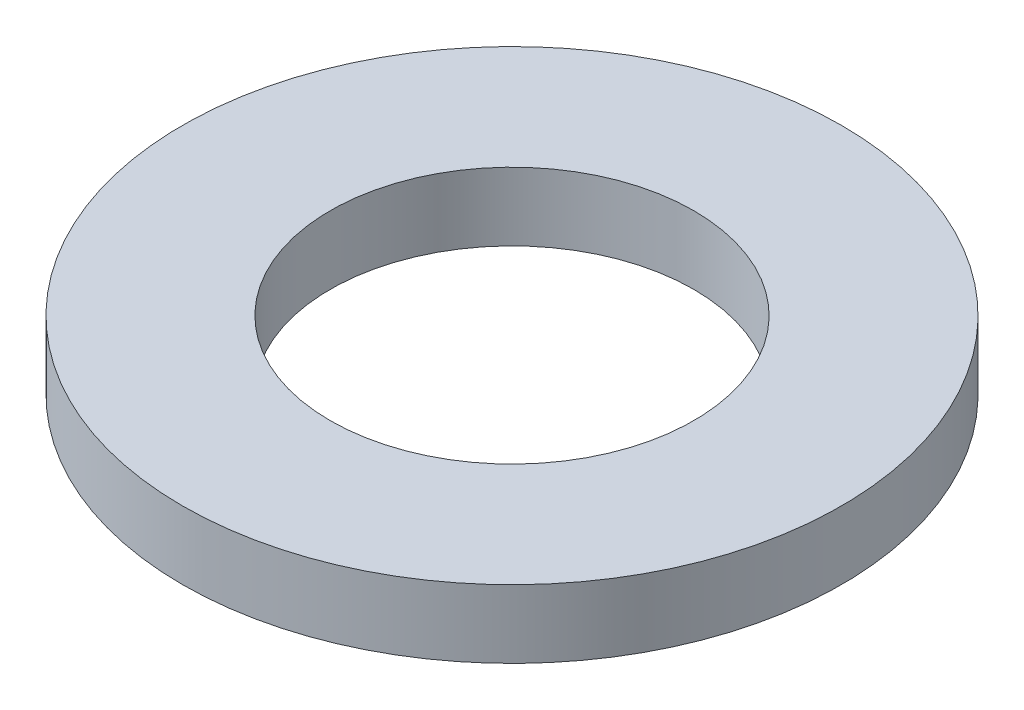
SolidWorks part; units mm, degrees
ref_plane "前视基准面" through (0, 0, 0) normal (0, 0, 1) x (1, 0, 0)
ref_plane "上视基准面" through (0, 0, 0) normal (0, 1, 0) x (1, 0, 0)
ref_plane "右视基准面" through (0, 0, 0) normal (1, 0, 0) x (0, 0, -1)
sketch "草图1" plane through (0, 0, 0) normal (0, 1, 0) x (1, 0, 0)
  circle A0 centre (0, 0) radius 5.8
  circle A1 centre (0, 0) radius 3.2
extrude "凸台-拉伸1" add sketch "草图1" along normal blind 1.2
